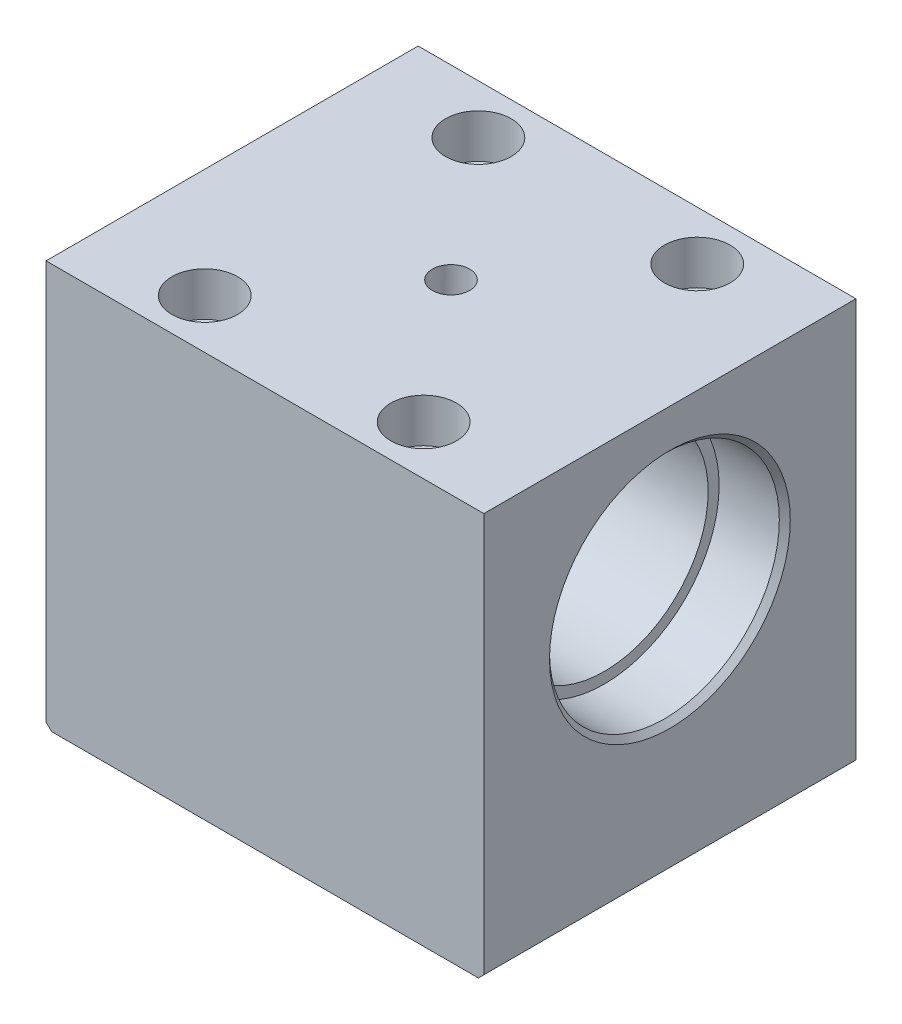
from build123d import *

# Parameters (mm, degrees)
SKETCH1_W                                            = 40
SKETCH1_H                                            = 68
BOSS_EXTRUDE1_DEPTH                                  = 37
M8_TAPPED_HOLE1_D                                    = 6.8
M8_TAPPED_HOLE1_DEPTH                                = 30
M8_TAPPED_HOLE1_TIP                                  = 2.042926105
SKETCH11_R                                           = 21
CUT_EXTRUDE4_DEPTH                                   = 12
SKETCH12_R                                           = 19
CUT_EXTRUDE5_DEPTH                                   = 85.551759296
CHAMFER1_SIZE                                        = 1
CHAMFER3_SIZE                                        = 1
HOLE_SIZE_PER_SOCKET_HEAD_CAP_SCREW_TYPE_D           = 8
HOLE_SIZE_PER_SOCKET_HEAD_CAP_SCREW_TYPE_CBORE_D     = 12
HOLE_SIZE_PER_SOCKET_HEAD_CAP_SCREW_TYPE_CBORE_DEPTH = 8
MIRROR5_COPY_1_D                                     = 8
MIRROR5_COPY_1_CBORE_D                               = 12
MIRROR5_COPY_1_CBORE_DEPTH                           = 8


with BuildPart() as part:
    # Sketch1 → Boss-Extrude1 (new, symmetric)
    with BuildSketch(Plane(origin=(0, 0, 0), x_dir=(1, 0, 0), z_dir=(0, 1, 0))):
        with Locations((20, 0)):
            Rectangle(SKETCH1_W, SKETCH1_H)
    extrude(amount=BOSS_EXTRUDE1_DEPTH, both=True)

    # Mirror2: part across plane


with BuildPart() as part_1:
    add(part.part)
    add(part.part.mirror(Plane(origin=(0, 37, 0), x_dir=(0, 0, 1), z_dir=(-1, 0, 0))))

    # M8 Tapped Hole1
    with Locations(Plane(origin=(0, 37, 0), x_dir=(1, 0, 0), z_dir=(0, 1, 0))):
        with Locations((0, 0)):
            Hole(M8_TAPPED_HOLE1_D / 2, depth=M8_TAPPED_HOLE1_DEPTH)
            with Locations((0, 0, -(M8_TAPPED_HOLE1_DEPTH + M8_TAPPED_HOLE1_TIP / 2))):  # 118° drill point
                Cone(0, M8_TAPPED_HOLE1_D / 2, M8_TAPPED_HOLE1_TIP, mode=Mode.SUBTRACT)

    # Sketch11 → Cut-Extrude4 (cut)
    with BuildSketch(Plane(origin=(40, 0, 0), x_dir=(0, 0, -1), z_dir=(1, 0, 0))):
        with Locations((0, 8)):
            Circle(SKETCH11_R)
    cut_extrude4 = extrude(amount=-CUT_EXTRUDE4_DEPTH, mode=Mode.SUBTRACT)

    # Mirror3: Cut-Extrude4 across plane
    add(cut_extrude4.mirror(Plane(origin=(0, 0, 0), x_dir=(0, 0, 1), z_dir=(1, 0, 0))), mode=Mode.SUBTRACT)

    # Sketch12 → Cut-Extrude5 (cut, through all)
    with BuildSketch(Plane(origin=(28, 0, 0), x_dir=(0, 0, -1), z_dir=(1, 0, 0))):
        with Locations((0, 8)):
            Circle(SKETCH12_R)
    extrude(amount=-CUT_EXTRUDE5_DEPTH, mode=Mode.SUBTRACT)

    # Chamfer1
    chamfer1_edges = [part_1.edges().sort_by_distance(p)[0] for p in [
        (40, 8, 21),
        (-40, 8, 21),
    ]]
    chamfer(chamfer1_edges, length=CHAMFER1_SIZE)

    # Chamfer3
    chamfer3_edges = [part_1.edges().sort_by_distance(p)[0] for p in [
        (-40, -37, 0),
        (40, -37, 0),
    ]]
    chamfer(chamfer3_edges, length=CHAMFER3_SIZE)

    # Hole size per socket head cap screw type1 (through all)
    with Locations(Plane(origin=(0, 37, 0), x_dir=(1, 0, 0), z_dir=(0, 1, 0))):
        with Locations((-20, -25)):
            hole_size_per_socket_head_cap_screw_type = CounterBoreHole(HOLE_SIZE_PER_SOCKET_HEAD_CAP_SCREW_TYPE_D / 2, HOLE_SIZE_PER_SOCKET_HEAD_CAP_SCREW_TYPE_CBORE_D / 2, HOLE_SIZE_PER_SOCKET_HEAD_CAP_SCREW_TYPE_CBORE_DEPTH)

    # Mirror4: Hole size per socket head cap screw type1 across plane
    add(hole_size_per_socket_head_cap_screw_type.mirror(Plane.XY), mode=Mode.SUBTRACT)

    # Mirror5: Hole size per socket head cap screw type1 across plane
    add(hole_size_per_socket_head_cap_screw_type.mirror(Plane(origin=(0, 0, 0), x_dir=(0, 0, 1), z_dir=(1, 0, 0))), mode=Mode.SUBTRACT)

    # Mirror5 copy 1 (through all)
    with Locations(Plane(origin=(0, 37, 0), x_dir=(-1, 0, 0), z_dir=(0, 1, 0))):
        with Locations((-20, -25)):
            CounterBoreHole(MIRROR5_COPY_1_D / 2, MIRROR5_COPY_1_CBORE_D / 2, MIRROR5_COPY_1_CBORE_DEPTH)


solid = part_1.part
